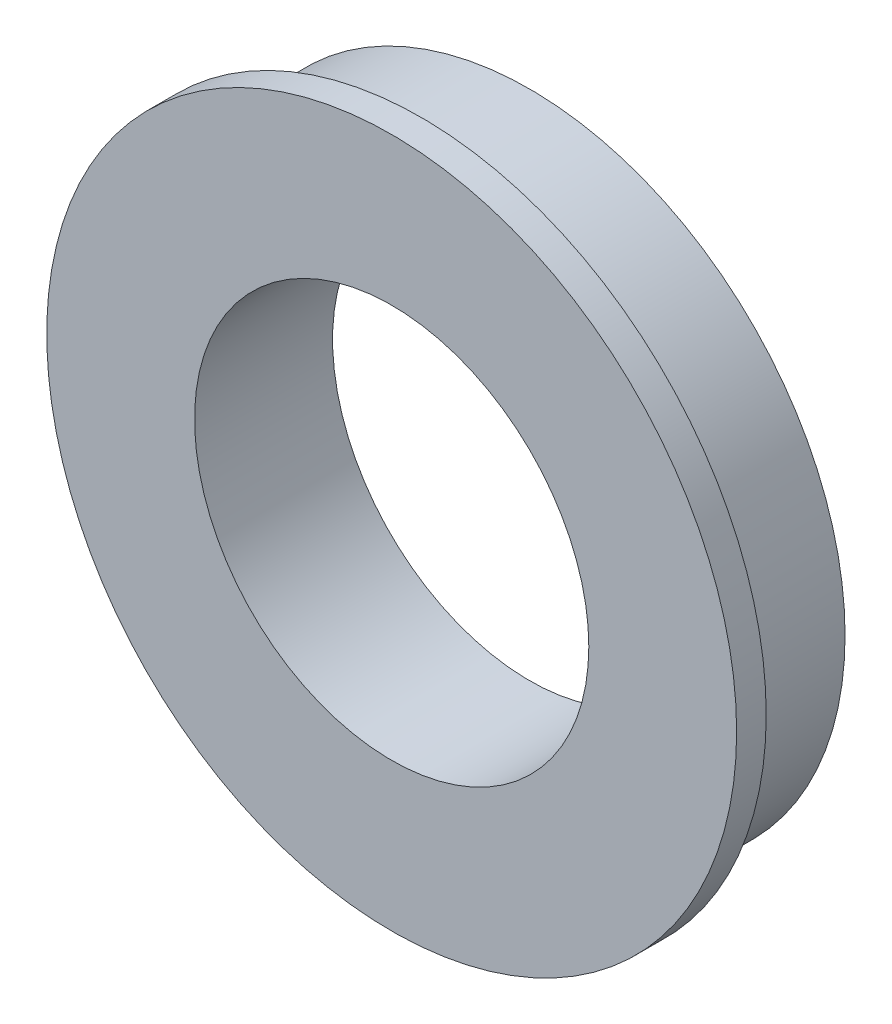
from build123d import *

# Parameters (mm, degrees)
SKETCH_1_R      = 16
SKETCH_1_R_2    = 10
EXTRUDE_1_DEPTH = 7
EXTRUDE_START   = -1.5
SKETCH_2_R      = 17.5
SKETCH_2_R_2    = 16
EXTRUDE_2_DEPTH = 1.5


with BuildPart() as part:
    # 草图1 → 凸台-拉伸1 (new body)
    with BuildSketch(Plane.XY):
        Circle(SKETCH_1_R)
        Circle(SKETCH_1_R_2, mode=Mode.SUBTRACT)
    extrude(amount=EXTRUDE_1_DEPTH)

    # 草图2 → 凸台-拉伸2 (add)
    with BuildSketch(Plane.XY.offset(7).offset(EXTRUDE_START)):
        Circle(SKETCH_2_R)
        Circle(SKETCH_2_R_2, mode=Mode.SUBTRACT)
    extrude(amount=EXTRUDE_2_DEPTH)


solid = part.part
